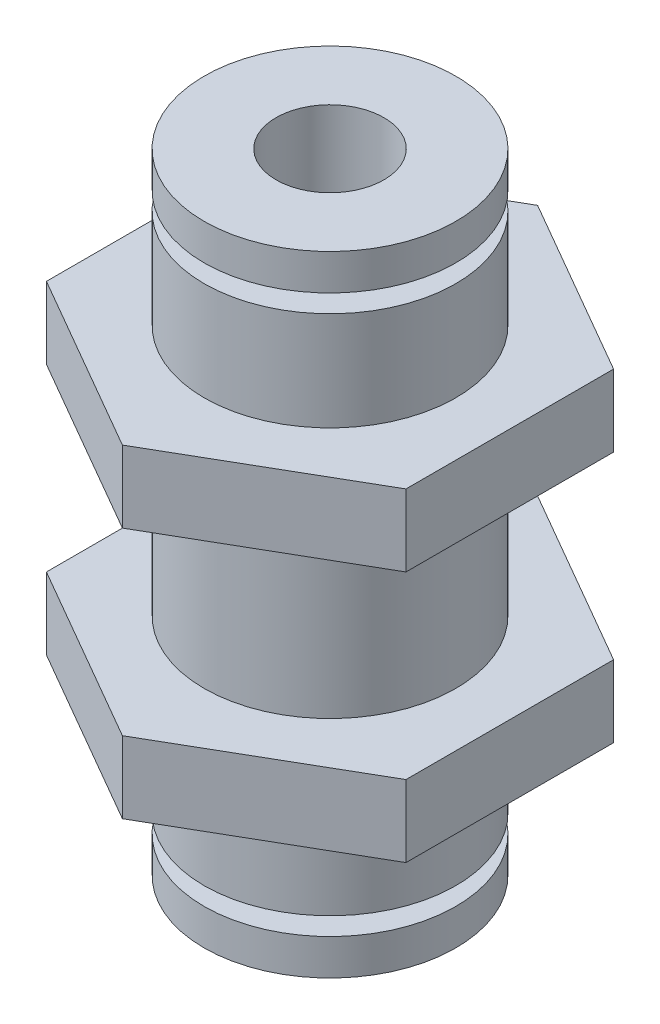
SolidWorks part; units mm, degrees
ref_plane "Front Plane" through (0, 0, 0) normal (0, 0, 1) x (1, 0, 0)
ref_plane "Top Plane" through (0, 0, 0) normal (0, 1, 0) x (1, 0, 0)
ref_plane "Right Plane" through (0, 0, 0) normal (1, 0, 0) x (0, 0, -1)
sketch "Sketch1" plane through (0, 0, 0) normal (0, 0, 1) x (1, 0, 0)
  line L0 (0, 17.5) -> (-7, 17.5)
  line L1 (-7, 17.5) -> (-7, 15.5)
  line L2 (-7, 15.5) -> (-5.5, 15.5)
  line L3 (-5.5, 15.5) -> (-5.5, 14.5)
  line L4 (-5.5, 14.5) -> (-7, 14.5)
  line L5 (-7, 14.5) -> (-7, -14.5)
  line L6 (0, 17.5) -> (0, -17.5)
  line L7 (0, -17.5) -> (-7, -17.5)
  line L8 (-7, -17.5) -> (-7, -15.5)
  line L9 (-7, -15.5) -> (-5.5, -15.5)
  line L10 (-5.5, -15.5) -> (-5.5, -14.5)
  line L11 (-5.5, -14.5) -> (-7, -14.5)
  dimension "D1" = 35
  dimension "D2" = 2
  dimension "D3" = 1
  dimension "D4" = 7
  dimension "D5" = 7
  dimension "D6" = 5.5
revolve "Revolve1" add sketch "Sketch1" angle 360 about L6
sketch "Sketch2" plane through (0, 17.5, 0) normal (0, 1, 0) x (1, 0, 0)
  circle A0 centre (0, 0) radius 3
  dimension "D1" = 6
extrude "Cut-Extrude1" cut sketch "Sketch2" against normal through all
ref_plane "Plane1" through (0, 5, 0) normal (0, 1, 0) x (1, 0, 0)
sketch "Sketch3" plane through (0, 5, 0) normal (0, 1, 0) x (1, 0, 0)
  line L1 (0, 11.547) -> (-10, 5.7735)
  line L2 (-10, 5.7735) -> (-10, -5.7735)
  line L3 (-10, -5.7735) -> (0, -11.547)
  line L4 (0, -11.547) -> (10, -5.7735)
  line L5 (10, -5.7735) -> (10, 5.7735)
  line L6 (10, 5.7735) -> (0, 11.547)
  circle A0 centre (0, 0) radius 10 construction
  circle A1 centre (0, 0) radius 7 construction
  circle A2 centre (0, 0) radius 7
  dimension "D1" = 20
extrude "Boss-Extrude1" add sketch "Sketch3" along normal blind 4 separate body
ref_plane "Plane2" through (0, -5, 0) normal (0, 1, 0) x (1, 0, 0)
sketch "Sketch4" plane through (0, -5, 0) normal (0, 1, 0) x (1, 0, 0)
  line L6 (0, 11.547) -> (-10, 5.7735)
  line L7 (-10, 5.7735) -> (-10, -5.7735)
  line L8 (-10, -5.7735) -> (0, -11.547)
  line L9 (0, -11.547) -> (10, -5.7735)
  line L10 (10, -5.7735) -> (10, 5.7735)
  line L11 (10, 5.7735) -> (0, 11.547)
  line L12 (0, 11.547) -> (-10, 5.7735)
  line L13 (-10, 5.7735) -> (-10, -5.7735)
  line L14 (-10, -5.7735) -> (0, -11.547)
  line L15 (0, -11.547) -> (10, -5.7735)
  line L16 (10, -5.7735) -> (10, 5.7735)
  line L17 (10, 5.7735) -> (0, 11.547)
  circle A1 centre (0, 0) radius 7
  circle A2 centre (0, 0) radius 7
  dimension "D1" = 0
  dimension "D2" = 0
extrude "Boss-Extrude2" add sketch "Sketch4" against normal blind 4
